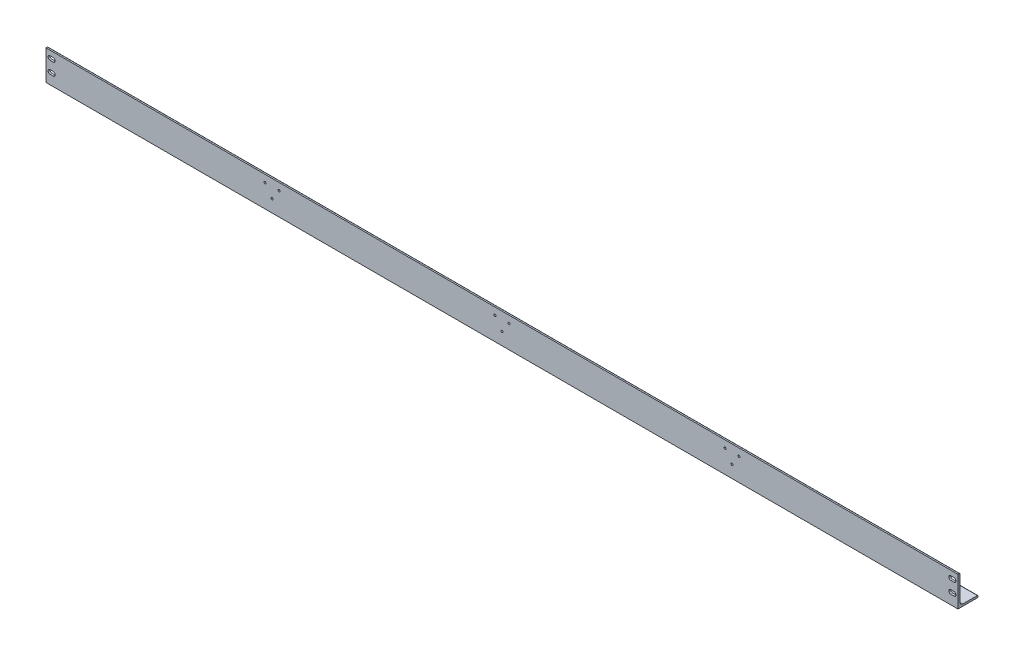
SolidWorks part; units mm, degrees
ref_plane "Front Plane" through (0, 0, 0) normal (0, 0, 1) x (1, 0, 0)
ref_plane "Top Plane" through (0, 0, 0) normal (0, 1, 0) x (1, 0, 0)
ref_plane "Right Plane" through (0, 0, 0) normal (1, 0, 0) x (0, 0, -1)
other "Configuration Table"
sketch "Sketch1" plane through (0, 0, 0) normal (0, 0, 1) x (1, 0, 0)
  line L0 (-1138, 0) -> (1138, 0)
  point P4 (0, 0)
  dimension "D1" = 2276
other "Unequal angle 7.5-5-5(1)"
ref_plane "Plane1" through (-1138, 0, 0) normal (1, 0, 0) x (0, 1, 0)
sketch "Sketch19" plane through (-1138, 0, 0) normal (1, 0, 0) x (0, 1, 0)
  line L0 (75, 0) -> (0, 0)
  line L1 (0, 0) -> (0, -50)
  line L2 (73.3333, -5) -> (13, -5)
  line L3 (5, -13) -> (5, -48.3333)
  line L4 (75, 0) -> (75, -3.3333)
  line L5 (0, -50) -> (3.3333, -50)
  arc A0 (75, -3.3333) -> (73.3333, -5) centre (73.3333, -3.3333) cw
  arc A1 (3.3333, -50) -> (5, -48.3333) centre (3.3333, -48.3333) ccw
  arc A2 (13, -5) -> (5, -13) centre (13, -13) ccw
  point P2 (0, -25)
  point P13 (37.5, 0)
  point P14 (0, 0)
  dimension "r1" = 1.6667
  dimension "r" = 8
  dimension "a" = 75
  dimension "d" = 5
  dimension "b" = 50
sketch "Sketch2" plane through (0, 5, 0) normal (0, 1, 0) x (1, 0, 0)
  line L0 (1138, 50) -> (-1138, 50) construction
  line L2 (1138, 50) -> (-1138, 50) construction
  arc A0 (-587.5, 29) -> (-595.5, 29) centre (-591.5, 29) ccw construction
  arc A1 (-13.5, 29) -> (-21.5, 29) centre (-17.5, 29) ccw construction
  arc A2 (560.5, 29) -> (552.5, 29) centre (556.5, 29) ccw construction
  point P0 (-591.5, 27)
  point P1 (-556.5, 27)
  point P3 (17.5, 27)
  point P5 (-17.5, 27)
  point P7 (591.5, 27)
  point P9 (556.5, 27)
  dimension "D1" = 23
  dimension "D2" = 23
  dimension "D3" = 35
  dimension "D4" = 0
  dimension "D5" = 35
  dimension "D6" = 0
  dimension "D7" = 23
  dimension "D8" = 35
  dimension "D9" = 23
  dimension "D10" = 0
  dimension "D11" = 23
  dimension "D12" = 23
hole_wizard "M6 Tapped Hole2" positions "Sketch2" profile "Sketch3" tap size "M6" standard "GB"
sketch "Sketch3" plane through (-591.5, 5, -27) normal (1, 0, 0) x (0, 0, 1)
  line L0 (0, 0) -> (0, 16.5022)
  line L1 (0, 16.5022) -> (2.5, 15)
  line L2 (2.5, 15) -> (2.5, 0)
  line L5 (2.5, 0) -> (0, 0)
  line L10 (0, 16.5022) -> (-2.5, 15) construction
  line L11 (0, -6.35) -> (0, 107.95) construction
  dimension "螺纹孔钻头直径" = 5
  dimension "螺纹孔钻头深度" = 15
  dimension "导头角度" = 118
cosmetic thread "Cosmetic thread 1" parameters "D1"=12, "D2"=6
cosmetic thread "Cosmetic thread 2" parameters "D1"=12, "D2"=6
cosmetic thread "Cosmetic thread 3" parameters "D1"=12, "D2"=6
cosmetic thread "Cosmetic thread 4" parameters "D1"=12, "D2"=6
cosmetic thread "Cosmetic thread 5" parameters "D1"=12, "D2"=6
cosmetic thread "Cosmetic thread 6" parameters "D1"=12, "D2"=6
sketch "Sketch10" plane through (0, 0, -5) normal (0, 0, -1) x (-1, 0, 0)
  line L0 (-560.5, 56.9326) -> (-552.5, 56.9326) construction
  line L1 (-560.5, 61.9326) -> (-560.5, 51.9326) construction
  line L2 (-552.5, 51.9326) -> (-552.5, 61.9326) construction
  line L3 (-587.5, 56.9326) -> (-595.5, 56.9326) construction
  line L4 (-587.5, 51.9326) -> (-587.5, 61.9326) construction
  line L5 (-595.5, 61.9326) -> (-595.5, 51.9326) construction
  line L6 (-578, 30.9326) -> (-570, 30.9326) construction
  line L7 (-578, 35.9326) -> (-578, 25.9326) construction
  line L8 (-570, 25.9326) -> (-570, 35.9326) construction
  line L9 (-21.5, 56.9326) -> (-13.5, 56.9326) construction
  line L10 (-21.5, 61.9326) -> (-21.5, 51.9326) construction
  line L11 (-13.5, 51.9326) -> (-13.5, 61.9326) construction
  line L12 (21.5, 56.9326) -> (13.5, 56.9326) construction
  line L13 (21.5, 51.9326) -> (21.5, 61.9326) construction
  line L14 (13.5, 61.9326) -> (13.5, 51.9326) construction
  line L15 (-4, 30.9326) -> (4, 30.9326) construction
  line L16 (-4, 35.9326) -> (-4, 25.9326) construction
  line L17 (4, 25.9326) -> (4, 35.9326) construction
  line L18 (552.5, 56.9326) -> (560.5, 56.9326) construction
  line L19 (552.5, 61.9326) -> (552.5, 51.9326) construction
  line L20 (560.5, 51.9326) -> (560.5, 61.9326) construction
  line L21 (587.5, 56.9326) -> (595.5, 56.9326) construction
  line L22 (587.5, 61.9326) -> (587.5, 51.9326) construction
  line L23 (595.5, 51.9326) -> (595.5, 61.9326) construction
  line L24 (570, 30.9326) -> (578, 30.9326) construction
  line L25 (570, 35.9326) -> (570, 25.9326) construction
  line L26 (578, 25.9326) -> (578, 35.9326) construction
  point P18 (-591.5, 56.9326)
  point P19 (-556.5, 56.9326)
  point P20 (-574, 30.9326)
  point P57 (556.5, 56.9326)
  point P58 (591.5, 56.9326)
  point P59 (574, 30.9326)
  point P60 (-17.5, 56.9326)
  point P61 (0, 30.9326)
  point P62 (17.5, 56.9326)
hole_wizard "M6 Tapped Hole1" positions "Sketch10" profile "Sketch11" tap size "M6" standard "GB"
sketch "Sketch11" plane through (-17.5, 56.9326, -5) normal (1, 0, 0) x (0, 1, 0)
  line L0 (0, 0) -> (0, 16.5022)
  line L1 (0, 16.5022) -> (2.5, 15)
  line L2 (2.5, 15) -> (2.5, 0)
  line L5 (2.5, 0) -> (0, 0)
  line L10 (0, 16.5022) -> (-2.5, 15) construction
  line L11 (0, -6.35) -> (0, 107.95) construction
  dimension "螺纹孔钻头直径" = 5
  dimension "螺纹孔钻头深度" = 15
  dimension "导头角度" = 118
cosmetic thread "Cosmetic thread 26" parameters "D1"=12, "D2"=6
cosmetic thread "Cosmetic thread 27" parameters "D1"=12, "D2"=6
cosmetic thread "Cosmetic thread 28" parameters "D1"=12, "D2"=6
cosmetic thread "Cosmetic thread 29" parameters "D1"=12, "D2"=6
cosmetic thread "Cosmetic thread 30" parameters "D1"=12, "D2"=6
cosmetic thread "Cosmetic thread 31" parameters "D1"=12, "D2"=6
cosmetic thread "Cosmetic thread 32" parameters "D1"=12, "D2"=6
cosmetic thread "Cosmetic thread 33" parameters "D1"=12, "D2"=6
cosmetic thread "Cosmetic thread 34" parameters "D1"=12, "D2"=6
sketch "Sketch12" plane through (0, 0, -5) normal (0, 0, -1) x (-1, 0, 0)
  line L0 (1128, 58) -> (1120, 58) construction
  line L1 (1128, 53) -> (1120, 53)
  line L2 (1128, 63) -> (1120, 63)
  line L3 (-1138, 75) -> (1138, 75) construction
  line L4 (1138, 13) -> (1138, 73.3333) construction
  line L5 (1120, 28) -> (1128, 28) construction
  line L6 (1120, 33) -> (1128, 33)
  line L7 (1120, 23) -> (1128, 23)
  line L8 (-1128, 58) -> (-1120, 58) construction
  line L9 (-1128, 63) -> (-1120, 63)
  line L10 (-1128, 53) -> (-1120, 53)
  line L11 (-1128, 28) -> (-1120, 28) construction
  line L12 (-1128, 33) -> (-1120, 33)
  line L13 (-1128, 23) -> (-1120, 23)
  line L14 (-1138, 13) -> (-1138, 73.3333) construction
  arc A0 (1128, 53) -> (1128, 63) centre (1128, 58) ccw
  arc A1 (1120, 63) -> (1120, 53) centre (1120, 58) ccw
  arc A2 (1120, 33) -> (1120, 23) centre (1120, 28) ccw
  arc A3 (1128, 23) -> (1128, 33) centre (1128, 28) ccw
  arc A4 (-1128, 63) -> (-1128, 53) centre (-1128, 58) ccw
  arc A5 (-1120, 53) -> (-1120, 63) centre (-1120, 58) ccw
  arc A6 (-1128, 33) -> (-1128, 23) centre (-1128, 28) ccw
  arc A7 (-1120, 23) -> (-1120, 33) centre (-1120, 28) ccw
  point P2 (1124, 58)
  point P13 (1124, 28)
  point P20 (-1124, 58)
  point P26 (-1124, 28)
  dimension "D1" = 17
  dimension "D2" = 14
  dimension "D3" = 14
  dimension "D4" = 8
  dimension "D5" = 8
  dimension "D6" = 10
  dimension "D7" = 10
  dimension "D8" = 10
  dimension "D9" = 10
  dimension "D10" = 8
  dimension "D11" = 8
  dimension "D12" = 14
  dimension "D13" = 14
  dimension "D14" = 30
extrude "Cut-Extrude1" cut sketch "Sketch12" against normal blind 10
sketch "Sketch6" plane through (0, 0, -5) normal (0, 0, -1) x (-1, 0, 0)
  line L0 (1132, 60) -> (1132, 30)
  line L13 (-1138, 75) -> (1138, 75) construction
  line L14 (0, 0) -> (0, 154.6516) construction
  line L15 (-1132, 60) -> (-1132, 30)
  dimension "D2" = 45
  dimension "D3" = 15
